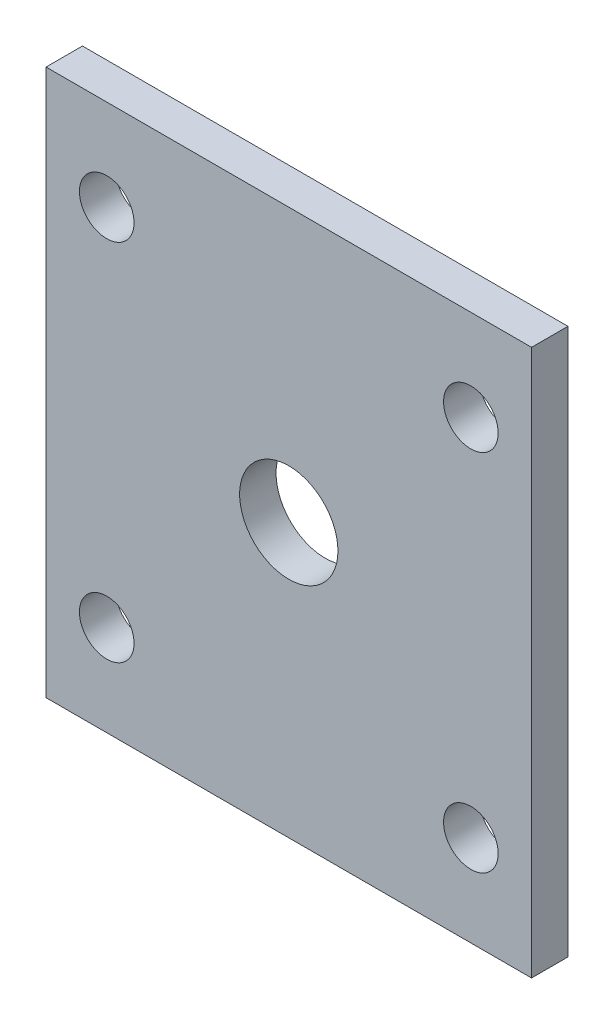
SolidWorks part; units mm, degrees
ref_plane "前视基准面" through (0, 0, 0) normal (0, 0, 1) x (1, 0, 0)
ref_plane "上视基准面" through (0, 0, 0) normal (0, 1, 0) x (1, 0, 0)
ref_plane "右视基准面" through (0, 0, 0) normal (1, 0, 0) x (0, 0, -1)
other "Configuration Table"
sketch "草图1" plane through (0, 0, 0) normal (0, 0, 1) x (1, 0, 0)
  line L0 (-40, -45) -> (40, -45)
  line L1 (40, -45) -> (40, 45)
  line L2 (40, 45) -> (-40, 45)
  line L3 (-40, 45) -> (-40, -45)
  point P0 (0, 0)
  dimension "D1" = 40
  dimension "D2" = 80
  dimension "D3" = 45
  dimension "D4" = 90
extrude "凸台-拉伸1" add sketch "草图1" against normal mid plane 6
sketch "草图2" plane through (0, 0, 0) normal (0, 0, 1) x (1, 0, 0)
  circle A0 centre (-30, -30) radius 4.5
  circle A1 centre (-30, 30) radius 4.5
  circle A2 centre (30, -30) radius 4.5
  circle A3 centre (30, 30) radius 4.5
  circle A4 centre (0, 0) radius 8.1
  point P0 (0, 0)
  dimension "D1" = 9
  dimension "D2" = 9
  dimension "D3" = 9
  dimension "D4" = 9
  dimension "D5" = 16.2
  dimension "D6" = 30
  dimension "D7" = 60
  dimension "D8" = 30
  dimension "D9" = 60
extrude "切除-拉伸1" cut sketch "草图2" against normal mid plane 26
